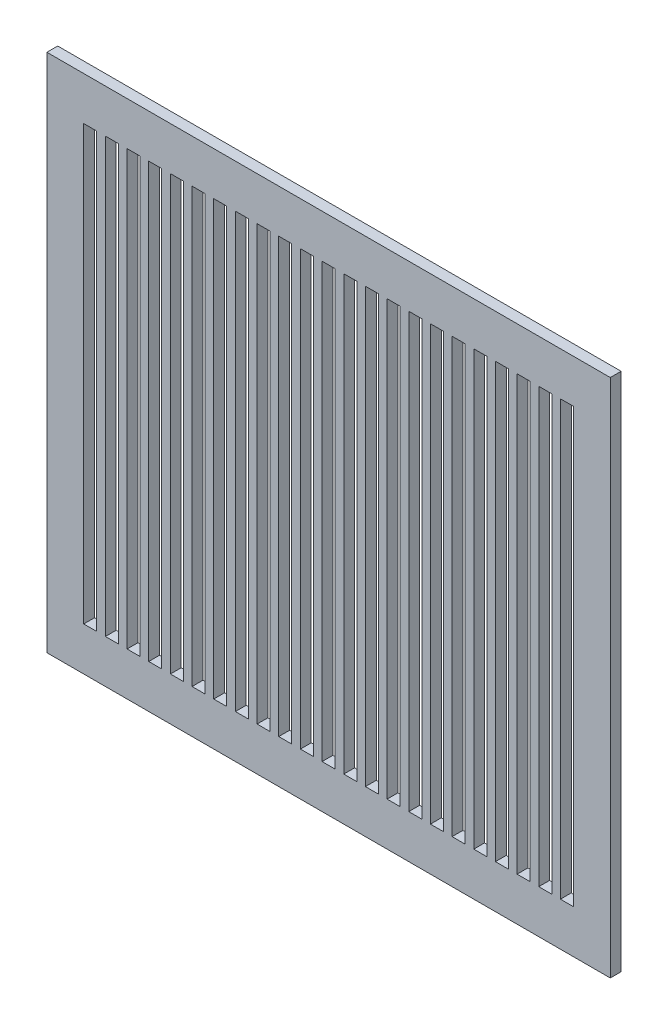
from build123d import *

# Parameters (mm, degrees)
SKETCH_1_W                 = 260
SKETCH_1_H                 = 240
EXTRUDE_1_DEPTH            = 5
SKETCH_2_W                 = 6
SKETCH_2_H                 = 200
CUT_EXTRUDE_1_DEPTH        = 177.988700204
PATTERN_LINEAR_1_COUNT     = 12
PATTERN_LINEAR_1_PITCH     = 10
PATTERN_LINEAR_1_COL_COUNT = 12
PATTERN_LINEAR_1_COL_PITCH = 10


with BuildPart() as part:
    # 草图1 → 凸台-拉伸1 (new body)
    with BuildSketch(Plane.XY):
        Rectangle(SKETCH_1_W, SKETCH_1_H)
    extrude(amount=EXTRUDE_1_DEPTH)

    # 草图2 → 切除-拉伸1 (cut, through all)
    with BuildSketch(Plane.XY.offset(5)):
        Rectangle(SKETCH_2_W, SKETCH_2_H)
    cut_extrude_1 = extrude(amount=-CUT_EXTRUDE_1_DEPTH, mode=Mode.SUBTRACT)

    # 阵列(线性)1: 切除-拉伸1 ×12
    with Locations(*[(i * PATTERN_LINEAR_1_PITCH, 0, 0) for i in range(1, PATTERN_LINEAR_1_COUNT)]):
        add(cut_extrude_1, mode=Mode.SUBTRACT)

    # 阵列(线性)1 col: 切除-拉伸1 ×12
    with Locations(*[(-i * PATTERN_LINEAR_1_COL_PITCH, 0, 0) for i in range(1, PATTERN_LINEAR_1_COL_COUNT)]):
        add(cut_extrude_1, mode=Mode.SUBTRACT)


solid = part.part
